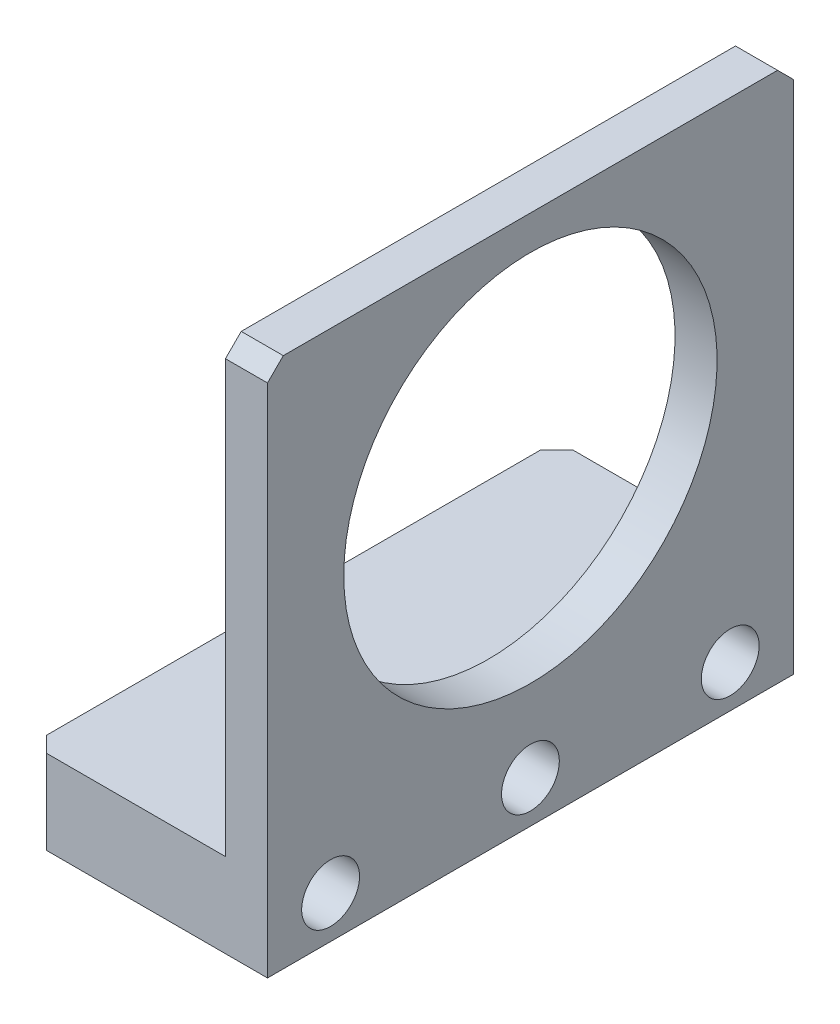
from build123d import *

# Parameters (mm, degrees)
EXTRUDE_1_DEPTH           = 50
CHAMFER_1_SIZE            = 3
CUT_EXTRUDE_1_REACH       = 138.711
SKETCH_3_R                = 35.5
HOLE_WIZARD_1_D           = 6.6
HOLE_WIZARD_1_CBORE_D     = 11
HOLE_WIZARD_1_CBORE_DEPTH = 35


with BuildPart() as part:
    # 草图2 → 凸台-拉伸1 (new, symmetric)
    with BuildSketch(Plane(origin=(409.637600706, 0.5, -34.379468655), x_dir=(1, 0, 0), z_dir=(0, 0, 1))):
        Polygon((-409.637600706, 100.5), (-409.637600706, -0.5), (-454.637600706, -0.5), (-454.637600706, 15.5), (-417.637600706, 15.5), (-417.637600706, 100.5), align=None)
    extrude(amount=EXTRUDE_1_DEPTH, both=True)

    # 倒角1
    chamfer_1_edges = [part.edges().sort_by_distance(p)[0] for p in [
        (-45, 8, 15.620531345),
        (-4, 101, 15.620531345),
        (-45, 8, -84.379468655),
        (-4, 101, -84.379468655),
    ]]
    chamfer(chamfer_1_edges, length=CHAMFER_1_SIZE)

    # 草图3 → 切除-拉伸1 (cut, up to next)
    with BuildSketch(Plane.ZY.offset(8), mode=Mode.PRIVATE) as cut_extrude_1_sk1:
        with Locations((-34.379468655, 59)):
            Circle(SKETCH_3_R)
    cut_extrude_1_tool1 = extrude(cut_extrude_1_sk1.sketch, amount=-CUT_EXTRUDE_1_REACH, mode=Mode.PRIVATE) & part.part
    add(cut_extrude_1_tool1.solids().sort_by_distance((-8, 59, -34.379469))[0], mode=Mode.SUBTRACT)

    # 打孔尺寸(%根据)内六角圆柱头螺钉的类型1 (through all)
    with Locations(Plane(origin=(0, 8, 3.620531345), x_dir=(0, 0, 1), z_dir=(1, 0, 0))):
        with Locations((0, 0), (-38, 0), (-76, 0)):
            CounterBoreHole(HOLE_WIZARD_1_D / 2, HOLE_WIZARD_1_CBORE_D / 2, HOLE_WIZARD_1_CBORE_DEPTH)


solid = part.part
